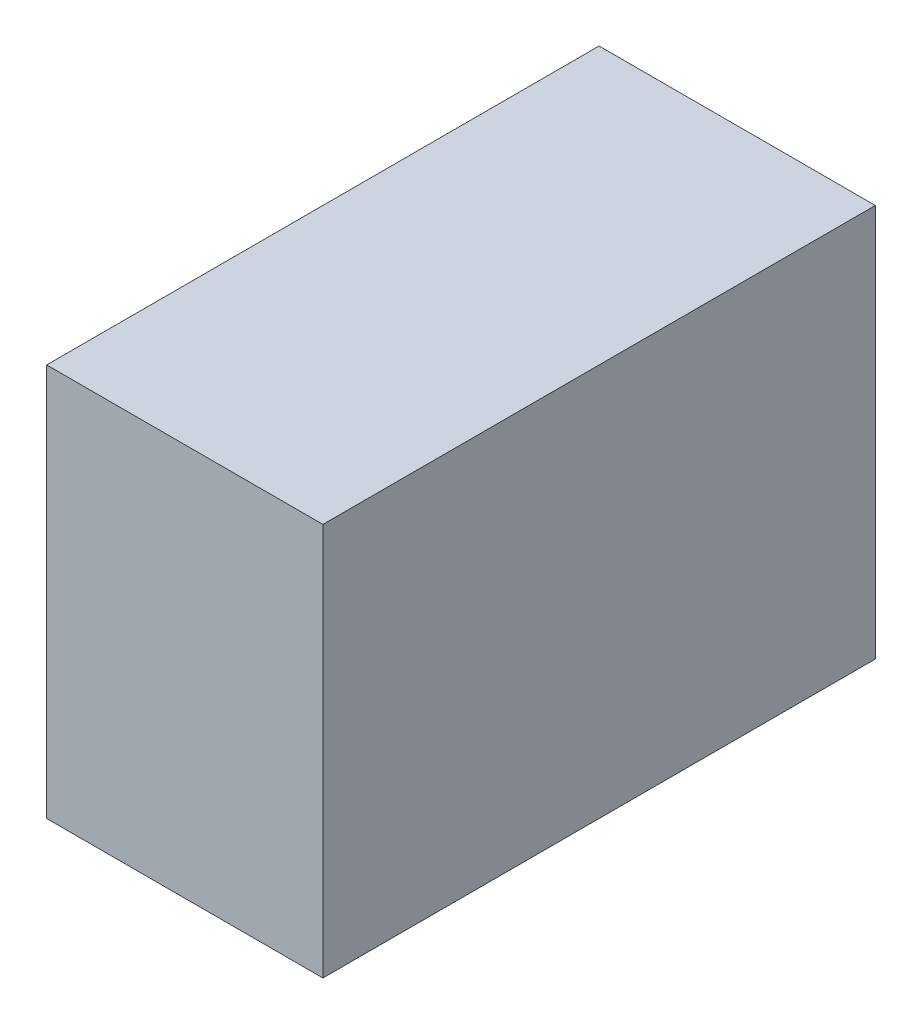
SolidWorks part; units mm, degrees
material "标准件"
ref_plane "前视基准面" through (0, 0, 0) normal (0, 0, 1) x (1, 0, 0)
ref_plane "上视基准面" through (0, 0, 0) normal (0, 1, 0) x (1, 0, 0)
ref_plane "右视基准面" through (0, 0, 0) normal (1, 0, 0) x (0, 0, -1)
sketch "草图1" plane through (0, 0, 0) normal (0, 1, 0) x (1, 0, 0)
  line L1 (-22.5, -45) -> (22.5, -45)
  line L2 (-22.5, -45) -> (-22.5, 45)
  line L3 (-22.5, 45) -> (22.5, 45)
  line L4 (22.5, -45) -> (22.5, 45)
  line L5 (-22.5, -45) -> (22.5, 45) construction
  line L6 (-22.5, 45) -> (22.5, -45) construction
  point P0 (0, 0)
  dimension "D1" = 90
  dimension "D2" = 45
extrude "凸台-拉伸1" add sketch "草图1" along normal blind 64
